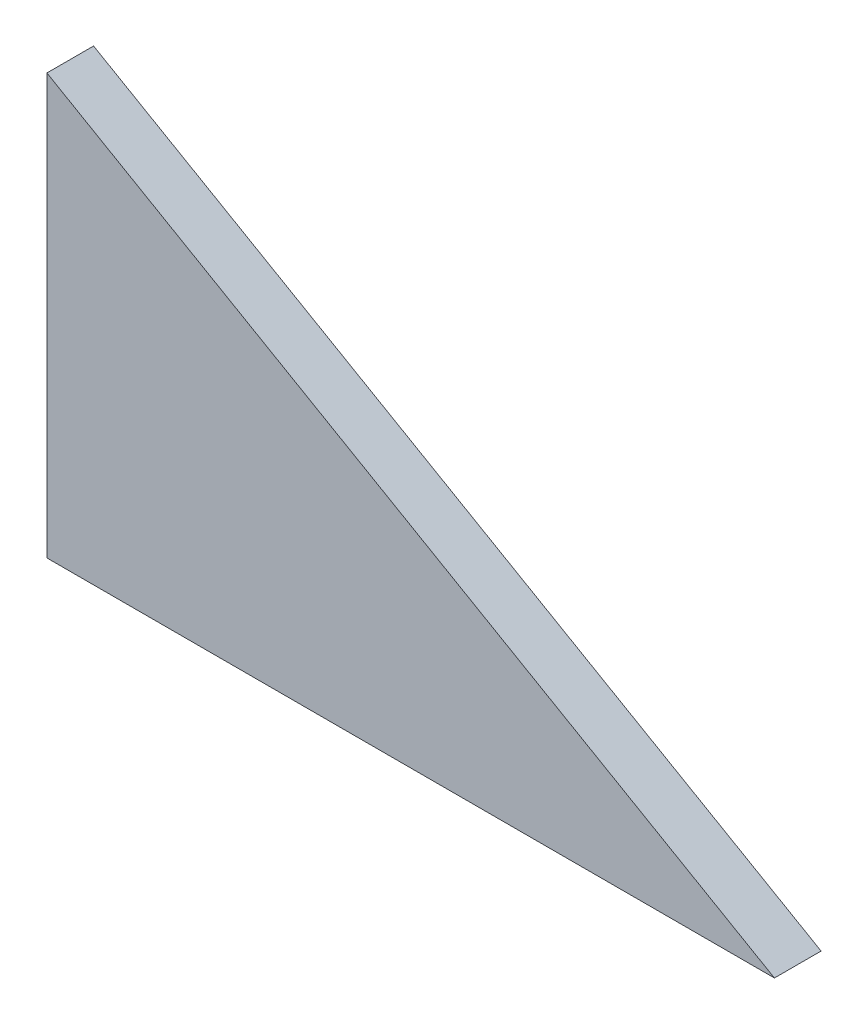
from build123d import *

# Parameters (mm, degrees)
BOSS_EXTRUDE1_DEPTH = 10


with BuildPart() as part:
    # Sketch1 → Boss-Extrude1 (new body)
    with BuildSketch(Plane.XY):
        Polygon((0, 0), (0, -90), (155.884572681, -90), align=None)
    extrude(amount=BOSS_EXTRUDE1_DEPTH)


solid = part.part
